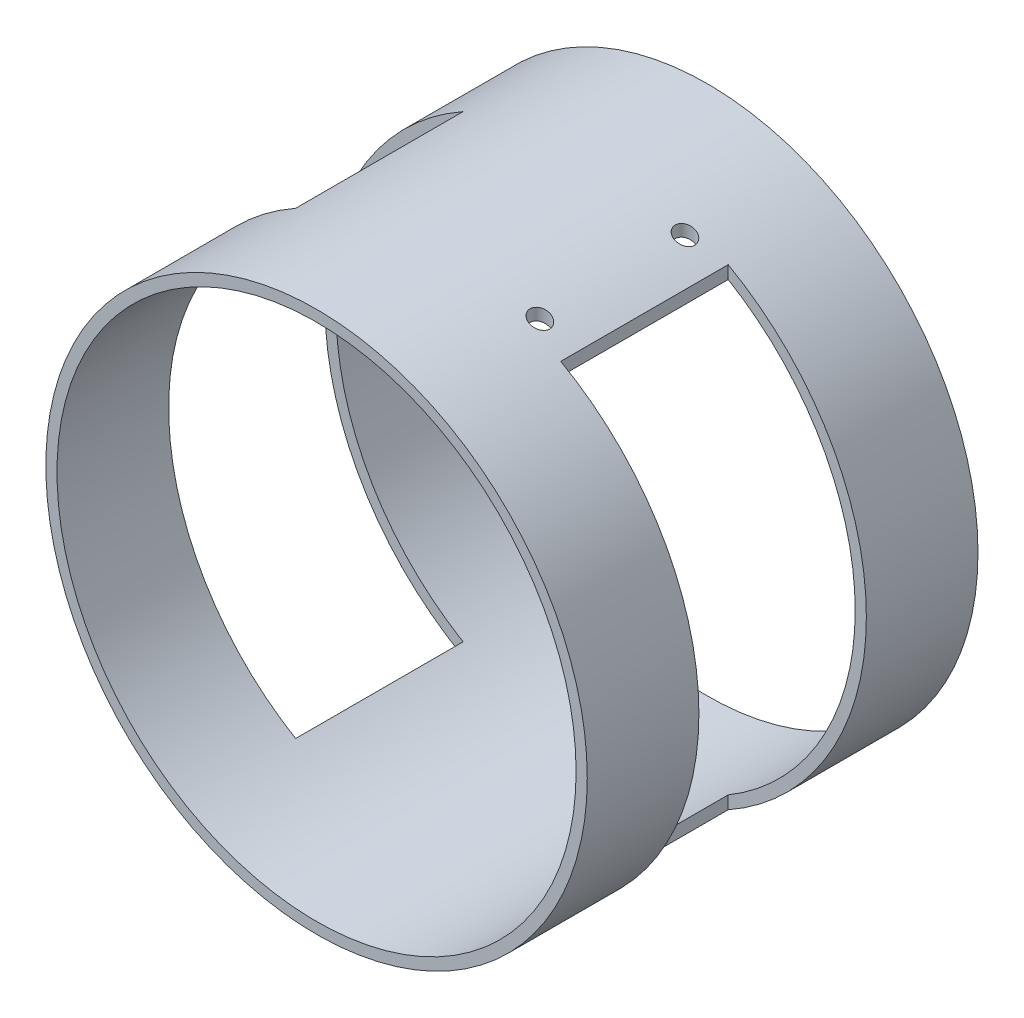
SolidWorks part; units mm, degrees
material "Q235"
ref_plane "Front Plane" through (0, 0, 0) normal (0, 0, 1) x (1, 0, 0)
ref_plane "Top Plane" through (0, 0, 0) normal (0, 1, 0) x (1, 0, 0)
ref_plane "Right Plane" through (0, 0, 0) normal (1, 0, 0) x (0, 0, -1)
sketch "Sketch1" plane through (0, 0, 0) normal (0, 0, 1) x (1, 0, 0)
  circle A0 centre (0, 0) radius 485
  circle A1 centre (0, 0) radius 465
  dimension "D1" = 970
  dimension "D2" = 930
extrude "Boss-Extrude1" add sketch "Sketch1" along normal blind 700
sketch "Sketch2" plane through (0, 0, 0) normal (0, 1, 0) x (1, 0, 0)
  line L0 (485, -200) -> (237.5, -200)
  line L1 (485, -700) -> (485, 0) construction
  line L2 (237.5, -200) -> (237.5, -500)
  line L3 (237.5, -500) -> (485, -500)
  line L4 (485, -500) -> (485, -200)
  line L5 (-485, -200) -> (-237.5, -200)
  line L6 (-237.5, -200) -> (-237.5, -500)
  line L7 (-237.5, -500) -> (-485, -500)
  line L8 (-485, -500) -> (-485, -200)
  line L9 (485, 0) -> (-485, 0) construction
  dimension "D1" = 475
  dimension "D2" = 237.5
  dimension "D3" = 247.5
  dimension "D4" = 300
  dimension "D5" = 200
extrude "Cut-Extrude1" cut sketch "Sketch2" against normal through all both and the other way through all
sketch "Sketch3" plane through (0, 0, 0) normal (0, 1, 0) x (1, 0, 0)
  line L0 (485, -200) -> (485, 0) construction
  line L1 (-485, -700) -> (485, -700) construction
  circle A0 centre (180, -220) radius 17.5
  circle A1 centre (180, -480) radius 17.5
  dimension "D1" = 35
  dimension "D2" = 305
  dimension "D3" = 220
  dimension "D4" = 220
extrude "Cut-Extrude2" cut sketch "Sketch3" along normal blind 700
sketch "Sketch4" plane through (0, 0, 0) normal (0, 1, 0) x (1, 0, 0)
  line L0 (-237.5, -350) -> (237.5, -350) construction
  line L1 (-237.5, -200) -> (-237.5, -500) construction
  line L2 (237.5, -500) -> (237.5, -200) construction
sketch "Sketch5" plane through (0, 0, 0) normal (1, 0, 0) x (0, 0, -1)
  line L0 (-734.9274, 0) -> (0, 0) construction
sketch "Sketch6" plane through (0, 0, 700) normal (0, 0, 1) x (1, 0, 0)
  line L0 (0, 0) -> (0, 485) construction
  circle A0 centre (0, 0) radius 485 construction
